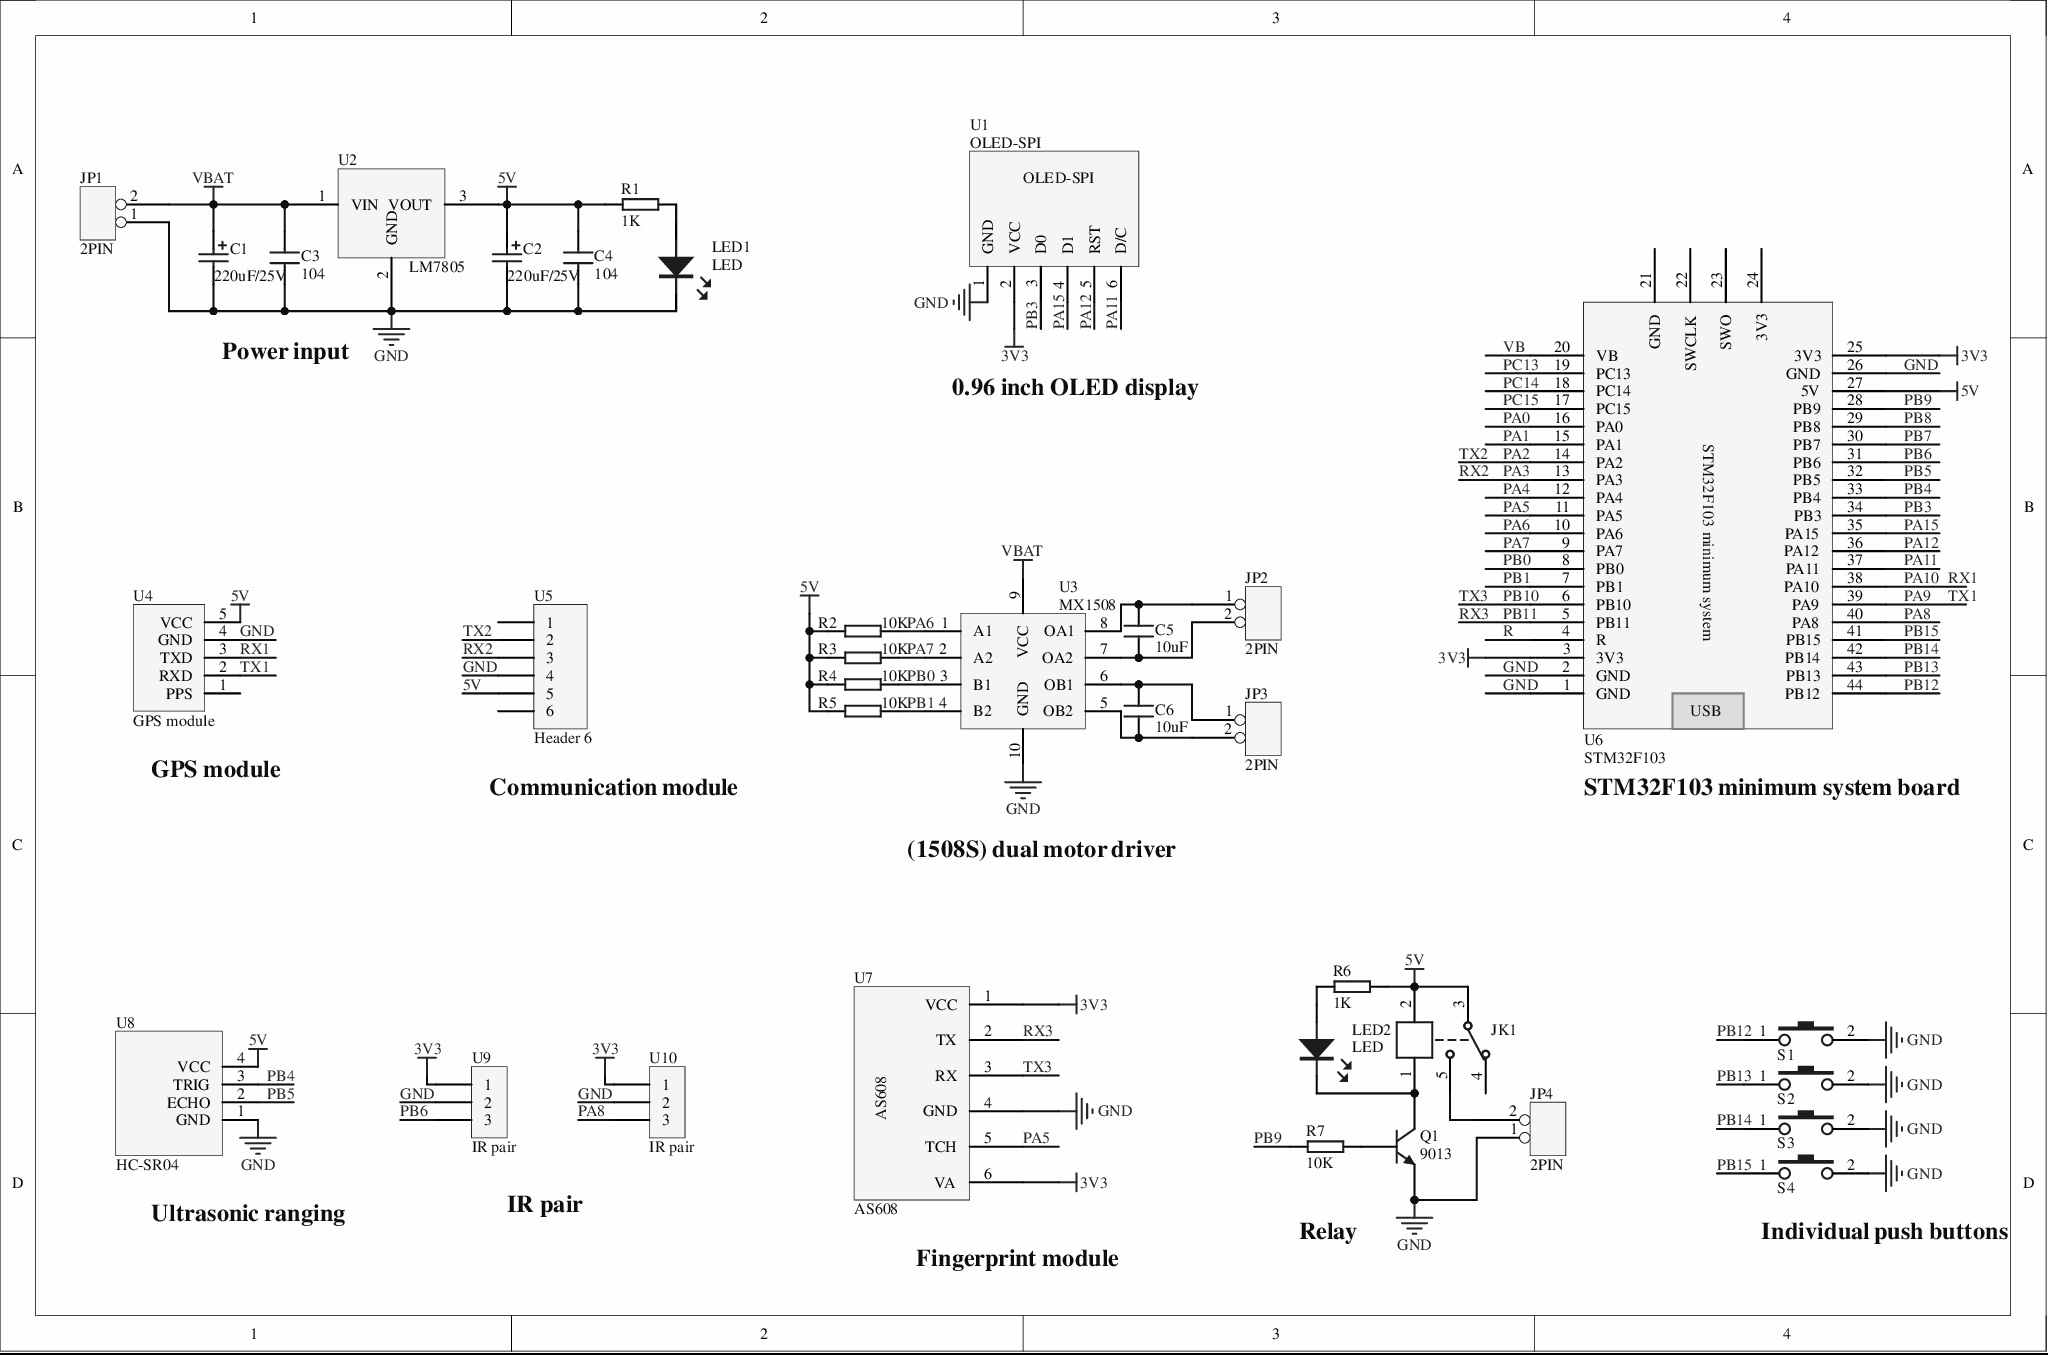
[diagram p0: MISC76356-3.SchDoc]
# Altium project MISC76356-2.PrjPcb
1 sheet, 35 parts. Net scope: global (net labels, ports and power ports of the same name join across sheets).
Board file: MISC76356.PcbDoc

## Sheet MISC76356-3.SchDoc
size A4

### Parts
C1  220uF/25V  [DIP-EC3.5X8X11.5]
C2  220uF/25V  [DIP-EC3.5X8X11.5]
C3  104  [RAD-0.2]
C4  104  [RAD-0.2]
C5  10uF  [0603C]
C6  10uF  [0603C]
JK1  SRD-05VDC-SL-C  [SRD-C_B]  (value not drawn)
JP1  2PIN  [XH2.54-LI-2P]
JP2  2PIN  [XH2.54-LI-2P]
JP3  2PIN  [XH2.54-LI-2P]
JP4  2PIN  [XH2.54-LI-2P]
LED1  LED  [LED 3MM-B]
LED2  LED  [LED 3MM-B]
Q1  9013  [TO-92A]
R1  1K  [AXIAL0.3]
R2  10K  [AXIAL0.3]
R3  10K  [AXIAL0.3]
R4  10K  [AXIAL0.3]
R5  10K  [AXIAL0.3]
R6  1K  [AXIAL0.3]
R7  10K  [AXIAL0.3]
S1  BUTTOM  [DIP-6X6X5]  (value not drawn)
S2  BUTTOM  [DIP-6X6X5]  (value not drawn)
S3  BUTTOM  [DIP-6X6X5]  (value not drawn)
S4  BUTTOM  [DIP-6X6X5]  (value not drawn)
U1  OLED-SPI  [OLED-SPI]
U2  LM7805  [TO220A]
U3  MX1508  [马达驱动芯片]
U4  GPS module  [GPS]
U5  Header 6  [Pin HDR1X6/2.54mm-S]
U6  STM32F103  [STM32FF103]
U7  AS608  [AS608]
U8  HC-SR04  [超声波MODE]
U9  IR pair  [火焰传感器]
U10  IR pair  [火焰传感器]

### Nets
3V3: U1.2(VCC) U6.3(3V3) U6.25(3V3) U7.1(VCC) U7.6(VA) U9.1 U10.1
5V: C2.1 C4.2 JK1.2 JK1.3 R1.2 R2.1 R3.1 R4.1 R5.1 R6.2 U2.3(VOUT) U4.5(VCC) U5.5 U6.27(5V) U8.4(VCC)
GND: C1.2 C2.2 C3.1 C4.1 JP1.1 JP4.1 LED1.2(K) Q1.E S1.2 S2.2 S3.2 S4.2 U1.1(GND) U2.2(GND) U3.10(GND) U4.4(GND) U5.4 U6.1(GND) U6.2(GND) U6.26(GND) U7.4(GND) U8.1(GND) U9.2 U10.2
VBAT: C1.1 C3.2 JP1.2 U2.1(VIN) U3.9(VCC)
PA0: U6.16(PA0)
PA1: U6.15(PA1)
PA2: U5.2 U6.14(PA2)  [also labelled TX2]
PA3: U5.3 U6.13(PA3)  [also labelled RX2]
PA4: U6.12(PA4)
PA5: U6.11(PA5) U7.5(TCH)
PA6: R2.2 U3.1(A1) U6.10(PA6)
PA7: R3.2 U3.2(A2) U6.9(PA7)
PA8: U6.40(PA8) U10.3
PA9: U4.2(RXD) U6.39(PA9)  [also labelled TX1]
PA10: U4.3(TXD) U6.38(PA10)  [also labelled RX1]
PA11: U1.6(D/C) U6.37(PA11)
PA12: U1.5(RST) U6.36(PA12)
PA15: U1.4(D1) U6.35(PA15)
PB0: R4.2 U3.3(B1) U6.8(PB0)
PB1: R5.2 U3.4(B2) U6.7(PB1)
PB3: U1.3(D0) U6.34(PB3)
PB4: U6.33(PB4) U8.3(TRIG)
PB5: U6.32(PB5) U8.2(ECHO)
PB6: U6.31(PB6) U9.3
PB7: U6.30(PB7)
PB8: U6.29(PB8)
PB9: R7.1 U6.28(PB9)
PB10: U6.6(PB10) U7.3(RX)  [also labelled TX3]
PB11: U6.5(PB11) U7.2(TX)  [also labelled RX3]
PB12: S1.1 U6.44(PB12)
PB13: S2.1 U6.43(PB13)
PB14: S3.1 U6.42(PB14)
PB15: S4.1 U6.41(PB15)
PC13: U6.19(PC13)
PC14: U6.18(PC14)
PC15: U6.17(PC15)
R: U6.4(R)
VB: U6.20(VB)
NetC5_1: C5.1 JP2.2 U3.7(OA2)
NetC5_2: C5.2 JP2.1 U3.8(OA1)
NetC6_1: C6.1 JP3.2 U3.5(OB2)
NetC6_2: C6.2 JP3.1 U3.6(OB1)
NetJK1_1: JK1.1 LED2.2(K) Q1.C
NetJK1_5: JK1.5 JP4.2
NetLED1_1: LED1.1(A) R1.1
NetLED2_1: LED2.1(A) R6.1
NetQ1_B: Q1.B R7.2

Not connected (* = marked no-connect by the designer): JK1 4; U4 1(PPS); U5 1 6; U6 21(GND) 22(SWCLK) 23(SWO) 24(3V3)

### Notes on the sheet
- Power input
- 0.96 inch OLED display
- (near U4) GPS module
- (near U5) Communication module
- (1508S) dual motor driver
- STM32F103 minimum system board
- IR pair
- Ultrasonic ranging
- (near U7) Fingerprint module
- Relay
- (near S4) Individual push buttons

### Library data of the parts
C1 C2 = Cap Pol2: Polarized Capacitor (Axial); Value: 100pF; Published: 8-Jun-2000; LatestRevisionDate: 17-Jul-2002; LatestRevisionNote: Re-released for DXP Platform.; PackageReference: POLAR0.8; PackageDescription: Polarized Capacitor; 2 Leads; Publisher: Altium Limited
C3-C6 = CAP: non-polarized capacitor
JK1 = SRD-05VDC-SL-C: 5V single-group converter
Q1 = 2N3904: NPN General Purpose Amplifier; Published: 8-Jun-2000; LatestRevisionDate: 15-Jan-2003; LatestRevisionNote: PCB Footprint 'BCY-W3/D4.7' replaced; DatasheetVersion: 1997; PackageVersion: Sep-1998; PackageReference: TO-92A; PackageDescription: TO, Flat Index; 3 In-Line, Axial Leads; Body Dia. 4.5mm; Leads 0.51 x 0.48 mm (max); ComponentLink1Description: Manufacturer Link; ComponentLink1URL: http://www.fairchildsemi.com/; ComponentLink2Description: Datasheet; ComponentLink2URL: http://www.fairchildsemi.com/ds/2N%2F2N3904.pdf; Publisher: Altium Limited
R1-R7 = RES: resistor
S1-S4 = BUTTOM: push button
U3 = 马达驱动模块: Motor driver module
U4 = GPS
U5 = Header 6: Header, 6-Pin; LatestRevisionDate: 17-Jul-2002; LatestRevisionNote: Re-released for DXP Platform.; Publisher: Altium Limited
U7 = 指纹模块
U8 = 超声波MODE: Ultrasonic module
U9 U10 = Pin HDR1X3